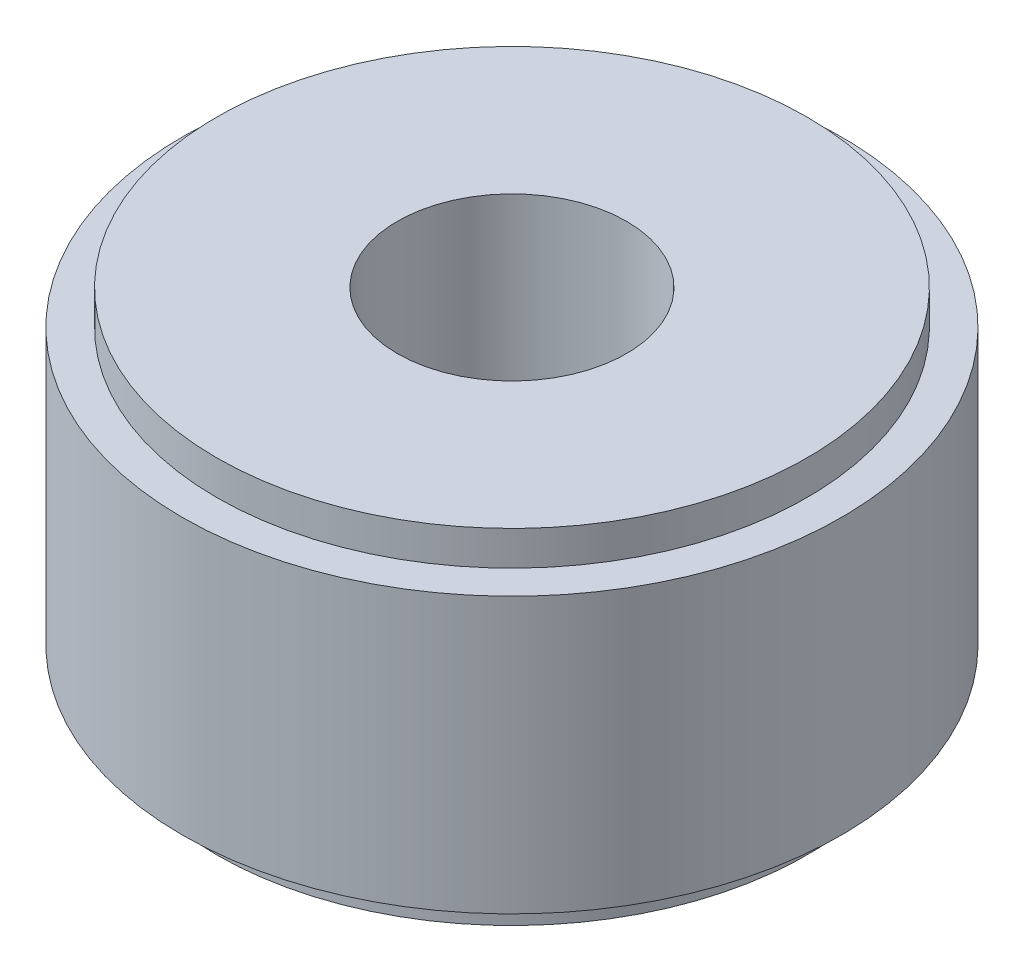
SolidWorks part; units mm, degrees
ref_plane "前视基准面" through (0, 0, 0) normal (0, 0, 1) x (1, 0, 0)
ref_plane "上视基准面" through (0, 0, 0) normal (0, 1, 0) x (1, 0, 0)
ref_plane "右视基准面" through (0, 0, 0) normal (1, 0, 0) x (0, 0, -1)
sketch "草图1" plane through (0, 0, 0) normal (0, 0, 1) x (1, 0, 0)
  line L0 (0, 27.5892) -> (0, -38.9455) construction
  line L1 (20, 9.7674) -> (20, -50.2326)
  line L2 (20, -50.2326) -> (51.5, -50.2326)
  line L3 (51.5, -50.2326) -> (51.5, -44.2326)
  line L4 (51.5, -44.2326) -> (57.5, -44.2326)
  line L5 (57.5, -44.2326) -> (57.5, 3.7674)
  line L6 (57.5, 3.7674) -> (51.5, 3.7674)
  line L7 (51.5, 3.7674) -> (51.5, 9.7674)
  line L8 (51.5, 9.7674) -> (20, 9.7674)
  dimension "D1" = 20
  dimension "D2" = 6
  dimension "D3" = 6
  dimension "D4" = 31.5
  dimension "D5" = 60
  dimension "D6" = 6
  dimension "D7" = 6
revolve "旋转1" add sketch "草图1" angle 360 about L0
